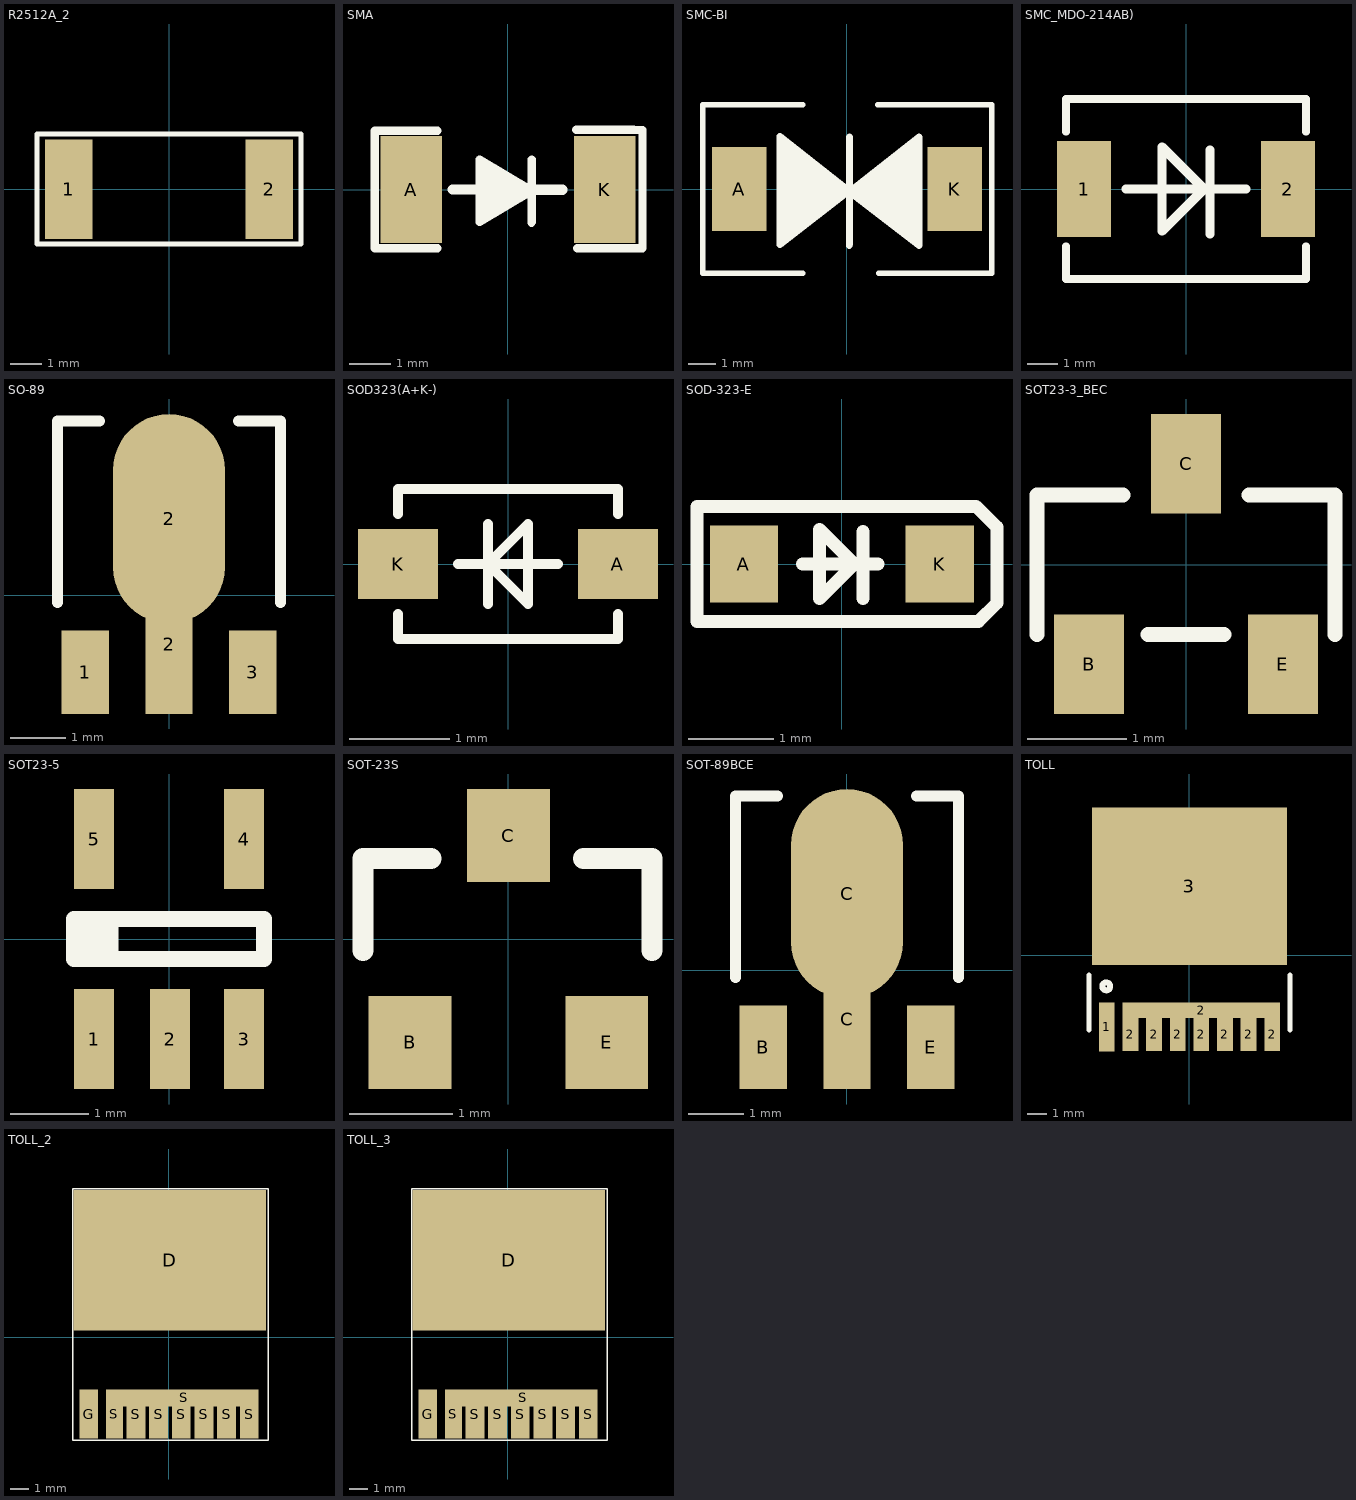
[diagram p0: the footprints below, top view; thin cyan lines are the x and y axes]
# Altium footprint library MISC86327.PcbLib: 30 footprints (part 2 of 2)
Each footprint in its own frame and in the unit in brackets; x right, y up, seen from the top. Pads: shape width x height; smd on the part's side, far side on the other; paste and mask are expansions set on the pad; w line width, h text height; cw(c..) or ccw(c..) is an arc to the next point about the centre after c.

## R2512A_2 [mm]
pads (2):
  rect 1.524x3.175 smd: 1(-3.2,0) 2(3.2,0)
Top Overlay:
  lines w0.152: -4.216,1.75 -4.216,-1.75 4.212,-1.75 4.212,1.75 ; -4.216,1.758 4.214,1.758
3D body "2512_R.step": height 0.64, standoff 0.02, extent -3.059,-1.594 3.241,1.606

## SMA [mm]
pads (2):
  rect 1.5x2.6 smd paste+0 mask+0: A(-2.35,0) K(2.35,0)
Top Overlay:
  lines w0.2: -3.24,-1.43 -3.02,-1.43 ; -3.24,-1.4 -3.24,1.41 ; -3.24,1.43 -2.97,1.43 ; 3.06,1.45 3.27,1.45 ; 3.06,-1.43 3.27,-1.43 ; 3.27,-1.42 3.27,1.43
  lines w0.203: -3.02,-1.43 -1.715,-1.43 ; -2.97,1.43 -1.715,1.43 ; -0.641,-0.665 -0.159,-0.182 ; -0.565,-0.538 -0.565,0.529 ; -0.438,-0.462 -0.438,0.453 ; -0.311,-0.462 -0.311,0.453 ; -0.159,-0.36 -0.159,0.351 ; -0.057,-0.36 0.299,-0.081 ; -0.032,-0.386 -0.032,0.326 0.299,-0.005 ; 0.095,-0.309 0.095,0.173 ; 0.572,-0.812 0.572,0.712 ; 0.578,-0.792 0.578,0.732 ; 1.664,1.455 3.06,1.45 ; 1.689,-1.43 3.06,-1.43 ; -0.692,-0.792 0.578,-0.03 -0.692,0.732 -0.692,-0.792
  lines w0.254: -1.35,0 0.6,0 ; 0.52,-0.01 1.32,-0.01
3D body: height 2.4, standoff 0, extent -2.3,-1.35 2.3,1.35

## SMC-BI [mm]
pads (2):
  rect 2x3.1 smd: A(-3.97,0) K(3.97,0)
Top Overlay:
  lines w0.127: -0.533,-0.12 0.465,-0.12 0.477,-0.108 -0.225,-0.108 -0.313,-0.02 -0.333,-0.02 -0.333,-0.01 -0.273,0.05 -0.223,0.05 -0.103,-0.07
  lines w0.203: -1.633,-3.099 -5.316,-3.1 -5.316,3.1 -1.633,3.099 ; 1.135,3.099 5.326,3.1 5.326,-3.1 1.161,-3.099
  lines w0.254: -2.296,-1.767 -2.296,1.662 -2.093,1.357 -2.093,-1.64 -1.89,-1.437 -1.89,1.357 -1.712,1.078 -1.712,-1.335 -1.509,-1.132 -1.509,-0.726 -1.509,1.001 -1.534,1.052 -1.28,0.773 -1.28,0.392 -1.305,-1.081 -1.051,-0.802 -1.077,-0.091 -1.102,0.697 ; -0.95,0.646 -0.924,-0.65 ; -0.848,0.544 -0.772,-0.573 ; -0.67,0.392 -0.645,-0.472 ; -0.518,0.341 -0.467,-0.421 ; -0.315,0.087 -0.289,-0.269 ; 0.041,-0.04 -2.474,1.941 -2.474,-2.047 0.092,-0.065 ; 0.082,-2.077 0.082,1.886 ; 0.082,-0.095 2.648,-2.077 2.648,1.911 0.133,-0.07 ; 0.092,-2.047 0.092,1.916 ; 0.463,-0.299 0.489,0.057 ; 0.641,-0.451 0.692,0.311 ; 0.819,-0.502 0.844,0.362 ; 0.946,-0.603 1.022,0.514 ; 1.098,-0.68 1.124,0.616 ; 1.276,0.667 1.251,-0.121 1.225,-0.832 1.479,-1.111 1.454,0.362 1.454,0.743 1.708,1.022 1.683,0.971 1.683,-0.756 1.683,-1.162 1.886,-1.365 1.886,1.048 2.064,1.327 2.064,-1.467 2.267,-1.67 2.267,1.327 2.47,1.632 2.47,-1.797

## SMC_MDO-214AB) [mm] "chip diode"
pads (2):
  rect 1.8x3.2 smd: 1(-3.4,0) 2(3.4,0)
Top Overlay:
  lines w0.254: -4,-1.905 -4,-3 4,-3 4,-1.905 ; -4,1.905 -4,3 4,3 4,1.905
  lines w0.3: -2,0 2,0 ; 0.8,-1.5 0.8,1.3 ; -0.8,-1.4 -0.8,1.4 0.6,0 -0.8,-1.4

## SO-89 [mil]
pads (4):
  rect 34x60 smd: 1(-60,-55) 3(60,-55)
  rect 34x100 smd: 2(0,-35)
  oval 80x150 smd: 2(0,55)
Top Overlay:
  lines w8: -80,-5 -80,125 -50,125 ; 50,125 80,125 80,-5

## SOD323(A+K-) [mm] "chip diode"
pads (2):
  rect 0.8x0.7 smd: A(1.1,0) K(-1.1,0)
Top Overlay:
  lines w0.1: -1.1,-0.5 -1.1,-0.75 1.1,-0.75 1.1,-0.5 ; -1.1,0.5 -1.1,0.75 1.1,0.75 1.1,0.5 ; -0.5,0 0.5,0 ; -0.2,-0.4 -0.2,0.4 ; -0.2,0 0.2,0.4 0.2,-0.4 -0.2,0

## SOD-323-E [mm]
pads (2):
  rect 0.8x0.9 smd: A(-1.15,0) K(1.15,0)
Top Overlay:
  lines w0.152: -0.464,0 0.425,0 ; 0.247,-0.406 0.247,-0.356 0.247,0.356 0.247,0.381 ; -1.7,-0.675 -1.7,0.675 1.577,0.675 1.822,0.432 1.822,-0.457 1.602,-0.675 -1.7,-0.675 ; -0.261,-0.406 -0.261,0.406 0.145,0 -0.261,-0.406
3D body "SOD-323.STEP": height 1, standoff 0, extent -1.3,-0.65 1.3,0.65

## SOT23-3_BEC [mm] "chip IC/MOS*"
pads (3):
  rect 0.7x1 smd: B(-0.975,-1) C(0,1.016) E(0.975,-1)
Top Overlay:
  lines w0.15: -1.5,-0.7 -1.5,0.7 -0.635,0.7 ; -0.381,-0.7 0.381,-0.7 ; 0.635,0.7 1.5,0.7 1.5,-0.7

## SOT23-5 [mil]
pads (5):
  rect 20x50 smd: 1(-37.5,-50) 2(0.5,-50) 3(37.5,-50) 4(37.5,50) 5(-37.5,50)
Top Overlay:
  rectangle: -46.41,-10.1 -25.31,9.9
  lines w8: -47.5,-10 47.5,-10 47.5,10 -47.5,10 -47.5,-10

## SOT-23S [mm]
pads (3):
  rect 0.8x0.9 smd: B(-0.95,-1) C(0,1) E(0.95,-1)
Top Overlay:
  lines w0.203: -1.407,-0.111 -1.407,0.778 -0.747,0.778 ; 0.726,0.778 1.387,0.778 1.387,-0.111
3D body "SOT-23-3.STEP": height 1.2, standoff 0, extent -1.45,-1.4 1.45,1.4

## SOT-89BCE [mil]
pads (4):
  rect 34x60 smd: B(-60,-55) E(60,-55)
  rect 34x100 smd: C(0,-35)
  oval 80x150 smd: C(0,55)
Top Overlay:
  lines w8: -80,-5 -80,125 -50,125 ; 50,125 80,125 80,-5

## TOLL [mm] "chip MOS"
height 3.35
pads (10):
  rect 0.8x2.5 smd: 1(-4.2,-3.638)
  rect 0.8x1.7 smd: 2(-3,-4) 2(-1.8,-4) 2(-0.6,-4) 2(0.6,-4) 2(1.8,-4) 2(3,-4) 2(4.2,-4)
  rect 8x0.8 smd: 2(0.6,-2.788)
  rect 9.9x8 smd: 3(0,3.5)
Top Overlay:
  circle w0.3: c-4.225,-1.575 r0.2
  lines w0.254: -5.1,-3.8 -5.1,-1 ; 5.1,-3.8 5.1,-1
Top Paste:
  region: -3.4,-4.85 -3.4,-3.25 -2.6,-3.25 -2.6,-4.85
  region: -2.2,-4.85 -2.2,-3.25 -1.4,-3.25 -1.4,-4.85
  region: -1,-4.85 -1,-3.25 -0.2,-3.25 -0.2,-4.85
  region: 0.2,-4.85 0.2,-3.25 1,-3.25 1,-4.85
  region: 1.4,-4.85 1.4,-3.25 2.2,-3.25 2.2,-4.85
  region: 2.6,-4.85 2.6,-3.25 3.4,-3.25 3.4,-4.85
  region: 3.8,-4.85 3.8,-3.25 4.6,-3.25 4.6,-4.85
  region: -4.6,-4.85 -4.6,-3.15 -3.8,-3.15 -3.8,-4.85
  region: -4.95,7.5 4.95,7.5 4.95,-0.5 -4.95,-0.5
  region: -3.4,-3.03 -3.4,-2.39 4.6,-2.39 4.6,-3.08

## TOLL_2 [mm]
pads (10):
  rect 10.2x7.45 smd: D(0.05,4.075)
  rect 1x2.61 smd: G(-4.25,-4.075) S(-1.75,-4.075) S(-0.55,-4.075) S(0.65,-4.075) S(1.85,-4.075) S(3.05,-4.075) S(4.25,-4.075)
  rect 0.9x2.61 smd: S(-2.9,-4.075)
  rect 7x0.9 smd: S(0.812,-3.22)
Top Overlay:
  lines w0.076: -5.106,-5.469 4.825,-5.469 5.257,-5.469 5.257,7.84 5.257,7.866 -5.106,7.866 -5.106,7.815 -5.106,-5.469

## TOLL_3 [mm]
pads (10):
  rect 10.2x7.45 smd: D(0.05,4.075)
  rect 1x2.61 smd: G(-4.25,-4.075) S(-1.75,-4.075) S(-0.55,-4.075) S(0.65,-4.075) S(1.85,-4.075) S(3.05,-4.075) S(4.25,-4.075)
  rect 0.9x2.61 smd: S(-2.9,-4.075)
  rect 7x0.9 smd: S(0.812,-3.22)
Top Overlay:
  lines w0.076: -5.106,-5.469 -5.106,7.815 -5.106,7.866 5.257,7.866 5.257,7.84 5.257,-5.469 4.825,-5.469 -5.106,-5.469